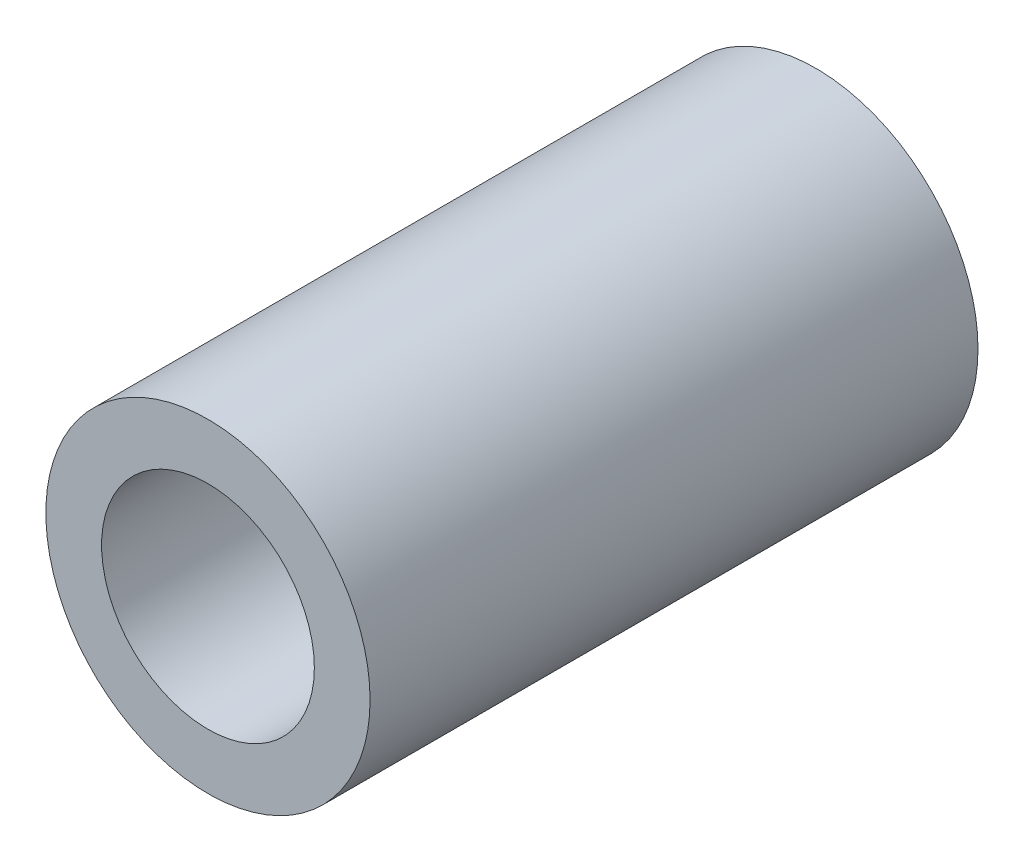
from build123d import *

# Parameters (mm, degrees)
SKETCH1_R                   = 8
BOSS_EXTRUDE1_DEPTH         = 30
M12X1_25_TAPPED_HOLE1_D     = 10.5
M12X1_25_TAPPED_HOLE1_DEPTH = 30
M12X1_25_TAPPED_HOLE1_TIP   = 3.15451825


with BuildPart() as part:
    # Sketch1 → Boss-Extrude1 (new body)
    with BuildSketch(Plane.XY):
        Circle(SKETCH1_R)
    extrude(amount=BOSS_EXTRUDE1_DEPTH)

    # M12x1.25 Tapped Hole1
    with Locations(Plane.XY.offset(30)):
        with Locations((0, 0)):
            Hole(M12X1_25_TAPPED_HOLE1_D / 2, depth=M12X1_25_TAPPED_HOLE1_DEPTH)
            with Locations((0, 0, -(M12X1_25_TAPPED_HOLE1_DEPTH + M12X1_25_TAPPED_HOLE1_TIP / 2))):  # 118° drill point
                Cone(0, M12X1_25_TAPPED_HOLE1_D / 2, M12X1_25_TAPPED_HOLE1_TIP, mode=Mode.SUBTRACT)


solid = part.part
